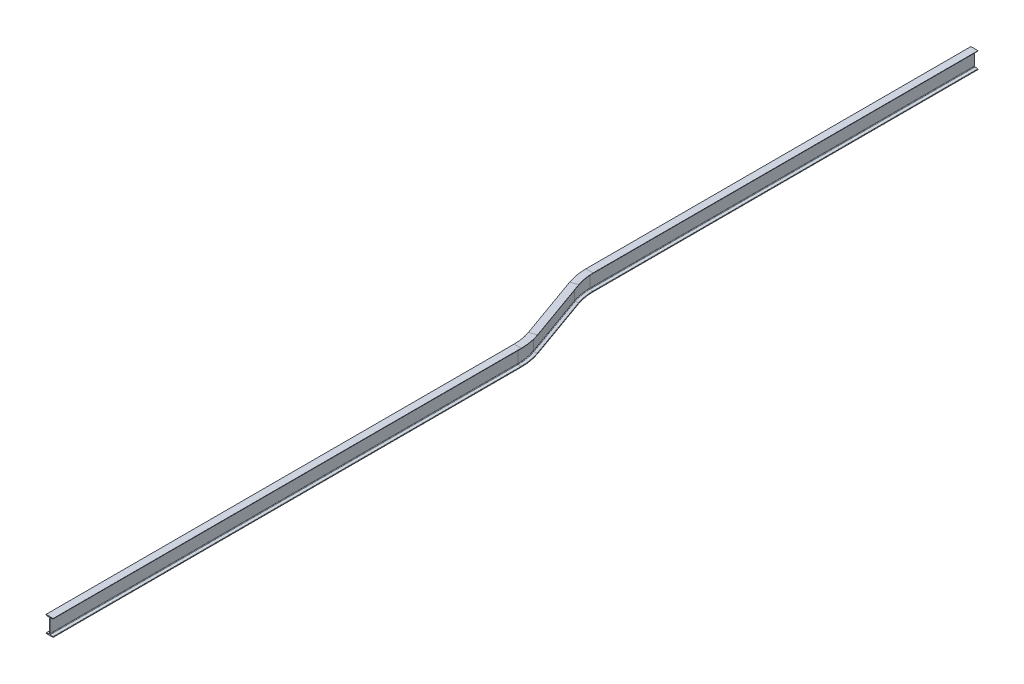
SolidWorks part; units mm, degrees
ref_plane "Front Plane" through (0, 0, 0) normal (0, 0, 1) x (1, 0, 0)
ref_plane "Top Plane" through (0, 0, 0) normal (0, 1, 0) x (1, 0, 0)
ref_plane "Right Plane" through (0, 0, 0) normal (1, 0, 0) x (0, 0, -1)
other "Configuration Table"
sketch "Sketch1" plane through (0, 0, 0) normal (0, 0, 1) x (1, 0, 0)
  line L24 (-61, 280) -> (-61, 276.2273)
  line L25 (-56.5713, 270.9994) -> (-13.0238, 263.7415)
  line L26 (-4.25, 253.3843) -> (-4.25, 26.6157)
  line L27 (-13.0238, 16.2585) -> (-56.5713, 9.0006)
  line L28 (-61, 3.7727) -> (-61, 0)
  line L29 (-61, 0) -> (61, 0)
  line L30 (61, 0) -> (61, 3.7727)
  line L31 (56.5713, 9.0006) -> (13.0238, 16.2585)
  line L32 (4.25, 26.6157) -> (4.25, 253.3843)
  line L33 (13.0238, 263.7415) -> (56.5713, 270.9994)
  line L34 (61, 276.2273) -> (61, 280)
  line L35 (61, 280) -> (-61, 280)
  arc A16 (-61, 276.2273) -> (-56.5713, 270.9994) centre (-55.7, 276.2273) ccw
  arc A17 (-4.25, 253.3843) -> (-13.0238, 263.7415) centre (-14.75, 253.3843) ccw
  arc A18 (-13.0238, 16.2585) -> (-4.25, 26.6157) centre (-14.75, 26.6157) ccw
  arc A19 (-56.5713, 9.0006) -> (-61, 3.7727) centre (-55.7, 3.7727) ccw
  arc A20 (61, 3.7727) -> (56.5713, 9.0006) centre (55.7, 3.7727) ccw
  arc A21 (4.25, 26.6157) -> (13.0238, 16.2585) centre (14.75, 26.6157) ccw
  arc A22 (13.0238, 263.7415) -> (4.25, 253.3843) centre (14.75, 253.3843) ccw
  arc A23 (56.5713, 270.9994) -> (61, 276.2273) centre (55.7, 276.2273) ccw
  dimension "D1" = 280
sketch "Sketch2" plane through (0, 0, 0) normal (0, 1, 0) x (1, 0, 0)
  line L0 (0, 0) -> (0, 7989.2885)
  line L1 (-54.6911, 8305.2446) -> (-445.3089, 9399.7554)
  line L2 (-500, 9715.7115) -> (-500, 16285)
  arc A0 (0, 7989.2885) -> (-54.6911, 8305.2446) centre (-940, 7989.2885) ccw
  arc A1 (-445.3089, 9399.7554) -> (-500, 9715.7115) centre (440, 9715.7115) cw
  point P7 (0, 8152)
  point P10 (-500, 9553)
  dimension "D5" = 940
  dimension "D1" = 16285
  dimension "D2" = 8152
  dimension "D3" = 500
  dimension "D4" = 6732
sweep "Sweep1" add profiles "Sketch1" path "Sketch2"
